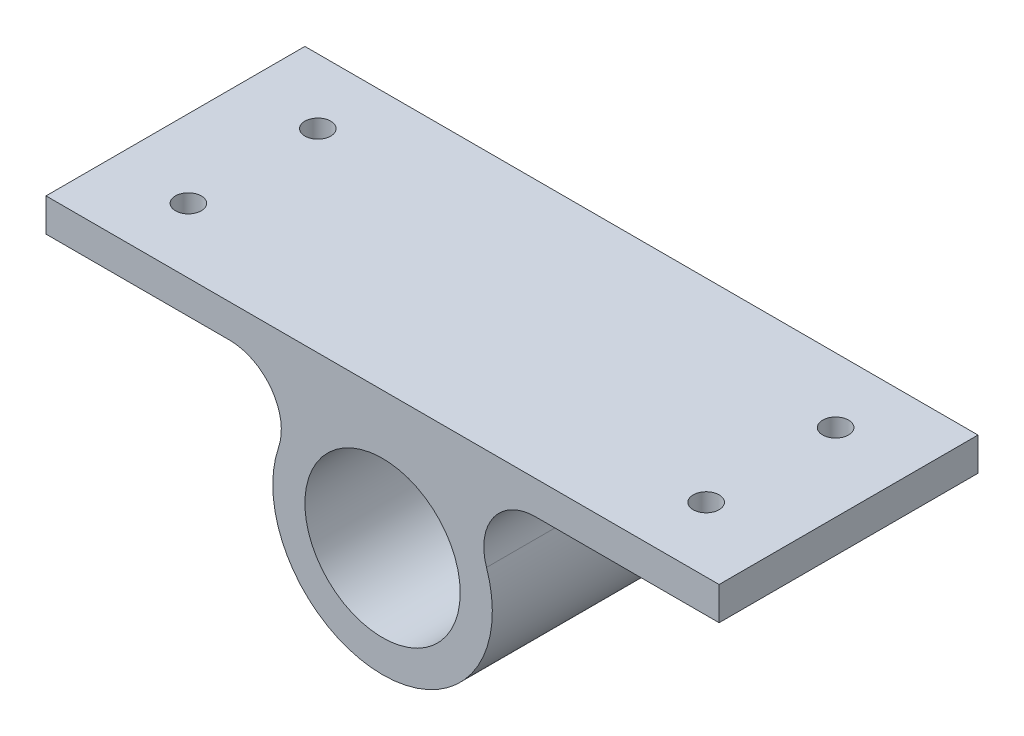
SolidWorks part; units mm, degrees
ref_plane "Front Plane" through (0, 0, 0) normal (0, 0, 1) x (1, 0, 0)
ref_plane "Top Plane" through (0, 0, 0) normal (0, 1, 0) x (1, 0, 0)
ref_plane "Right Plane" through (0, 0, 0) normal (1, 0, 0) x (0, 0, -1)
sketch "Sketch1" plane through (0, 0, 0) normal (0, 0, 1) x (1, 0, 0)
  line L0 (0, 144.1993) -> (0, -136.512) construction
  line L1 (325, 132) -> (-325, 132)
  line L2 (-325, 132) -> (-325, 100)
  line L3 (-325, 100) -> (-147.7701, 100)
  line L4 (325, 100) -> (147.7701, 100)
  line L5 (325, 132) -> (325, 100)
  circle A0 centre (0, 0) radius 75
  arc A1 (-100.4079, 33.9744) -> (100.4079, 33.9744) centre (0, 0) ccw
  arc A2 (-100.4079, 33.9744) -> (-147.7701, 100) centre (-147.7701, 50) ccw
  arc A3 (100.4079, 33.9744) -> (147.7701, 100) centre (147.7701, 50) cw
  point P14 (0, 132)
  dimension "D1" = 150
  dimension "D2" = 212
  dimension "D6" = 50
  dimension "D3" = 325
  dimension "D4" = 32
  dimension "D5" = 132
extrude "Boss-Extrude1" add sketch "Sketch1" along normal blind 250
sketch "Sketch2" plane through (0, 132, 0) normal (0, 1, 0) x (1, 0, 0)
  line L0 (0, 0) -> (0, -250) construction
  line L1 (-325, -125) -> (325, -125) construction
  line L2 (-325, -250) -> (-325, 0) construction
  line L3 (325, -250) -> (325, 0) construction
  line L4 (325, -250) -> (-325, -250) construction
  line L5 (325, 0) -> (-325, 0) construction
  circle A0 centre (-250, -62.5) radius 12.5
  circle A1 centre (-250, -187.5) radius 12.5
  circle A2 centre (250, -187.5) radius 12.5
  circle A3 centre (250, -62.5) radius 12.5
  dimension "D1" = 25
  dimension "D2" = 75
  dimension "D3" = 62.5
  dimension "D4" = 125
  dimension "D5" = 500
extrude "Cut-Extrude1" cut sketch "Sketch2" against normal up to next
